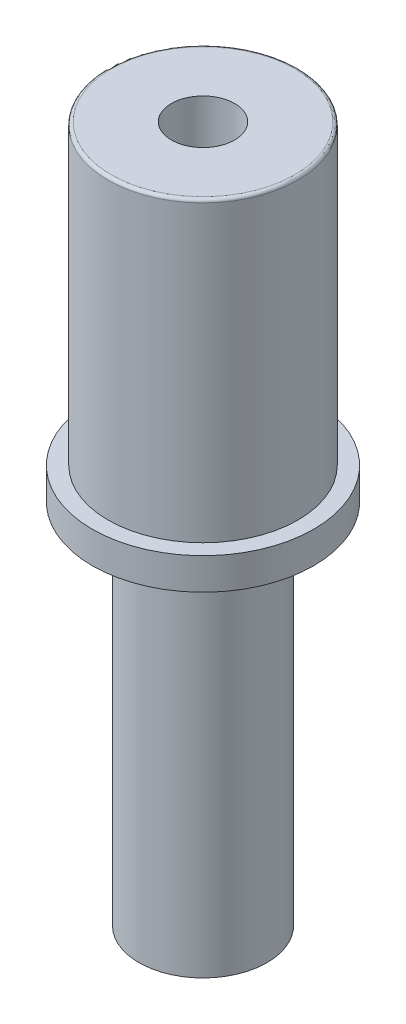
from build123d import *

# Parameters (mm, degrees)
FILLET3_R = 0.1


with BuildPart() as part:
    # Sketch1 → Revolve1 (revolve)
    with BuildSketch(Plane.XY, mode=Mode.PRIVATE) as revolve1_sk:
        Polygon((-3.5, 0), (-2.02328752, 0), (-2.02328752, -11.6), (-1, -11.6), (-1, 10.4), (-3, 10.4), (-3, 1), (-3.5, 1), align=None)
    revolve(revolve1_sk.sketch.rotate(Axis((0, -19.747048695, 0), (0, 1, 0)), 270), axis=Axis((0, -19.747048695, 0), (0, 1, 0)))

    # Fillet3
    fillet3_edges = [part.edges().sort_by_distance(p)[0] for p in [
        (0, 10.4, 3),
    ]]
    fillet(fillet3_edges, radius=FILLET3_R)


solid = part.part
